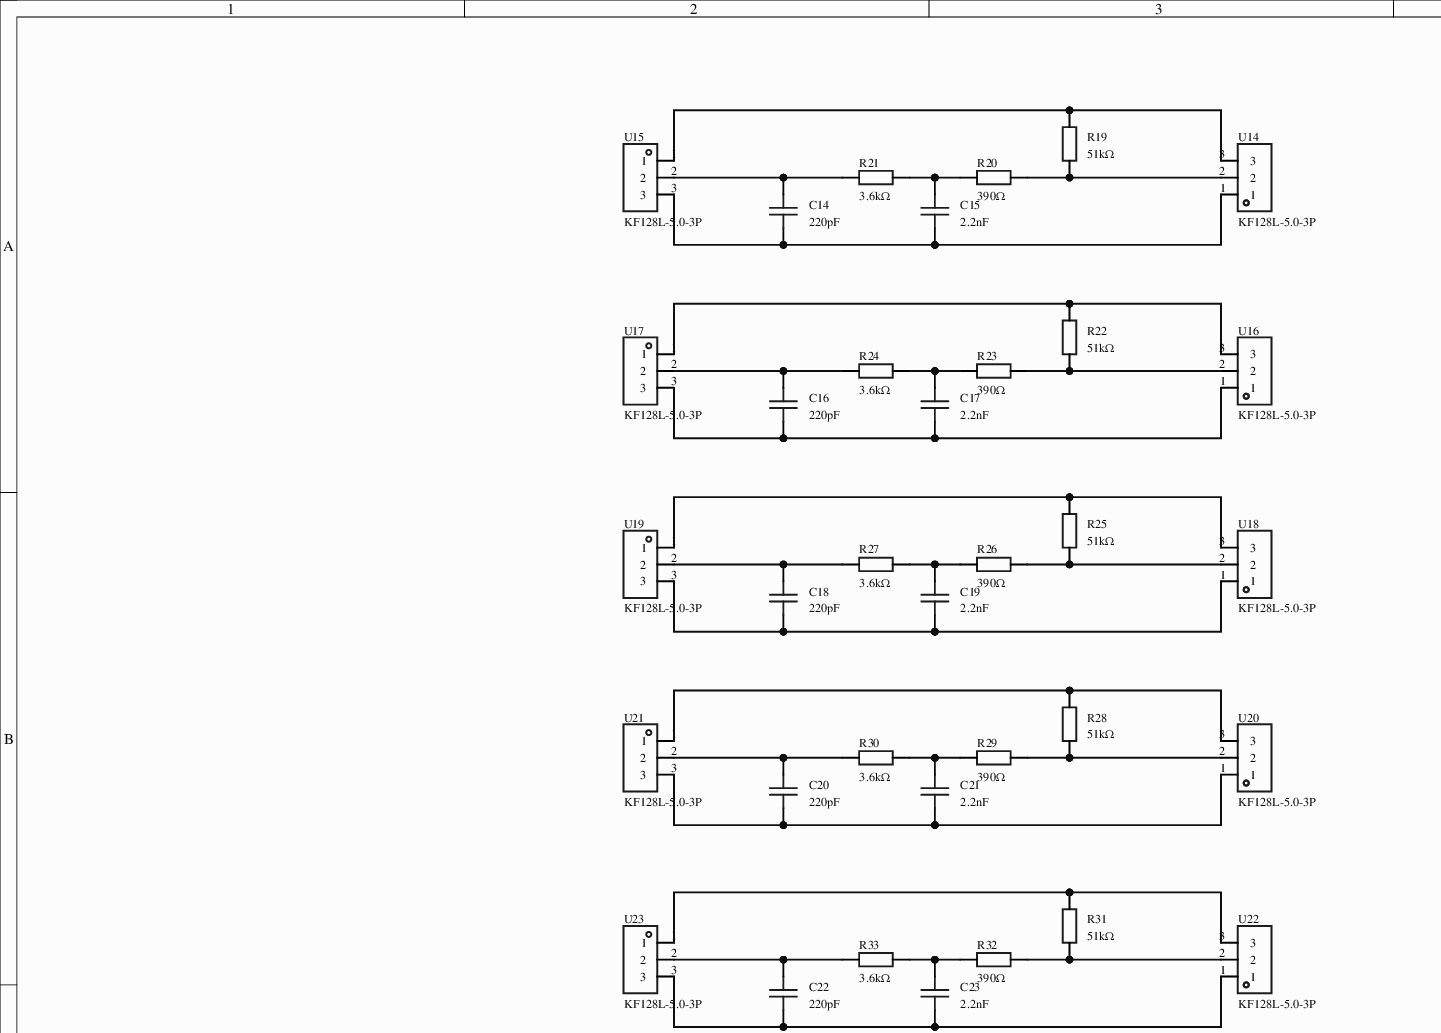
[diagram p0: MISC52118-3.schdoc, top left]
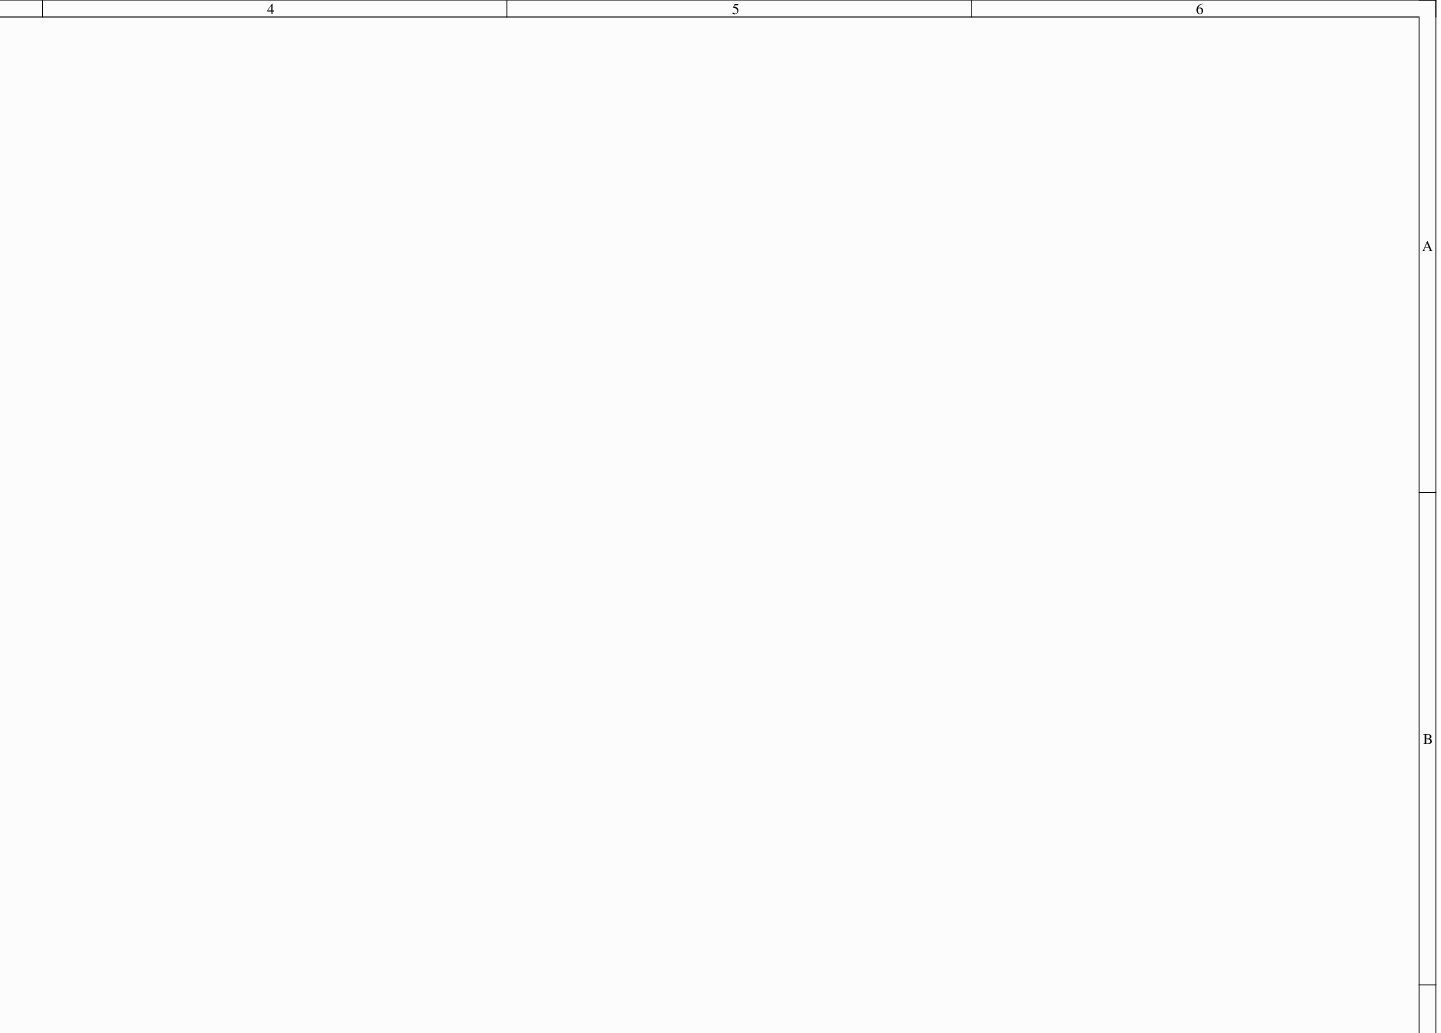
[diagram p1: MISC52118-3.schdoc, top right]
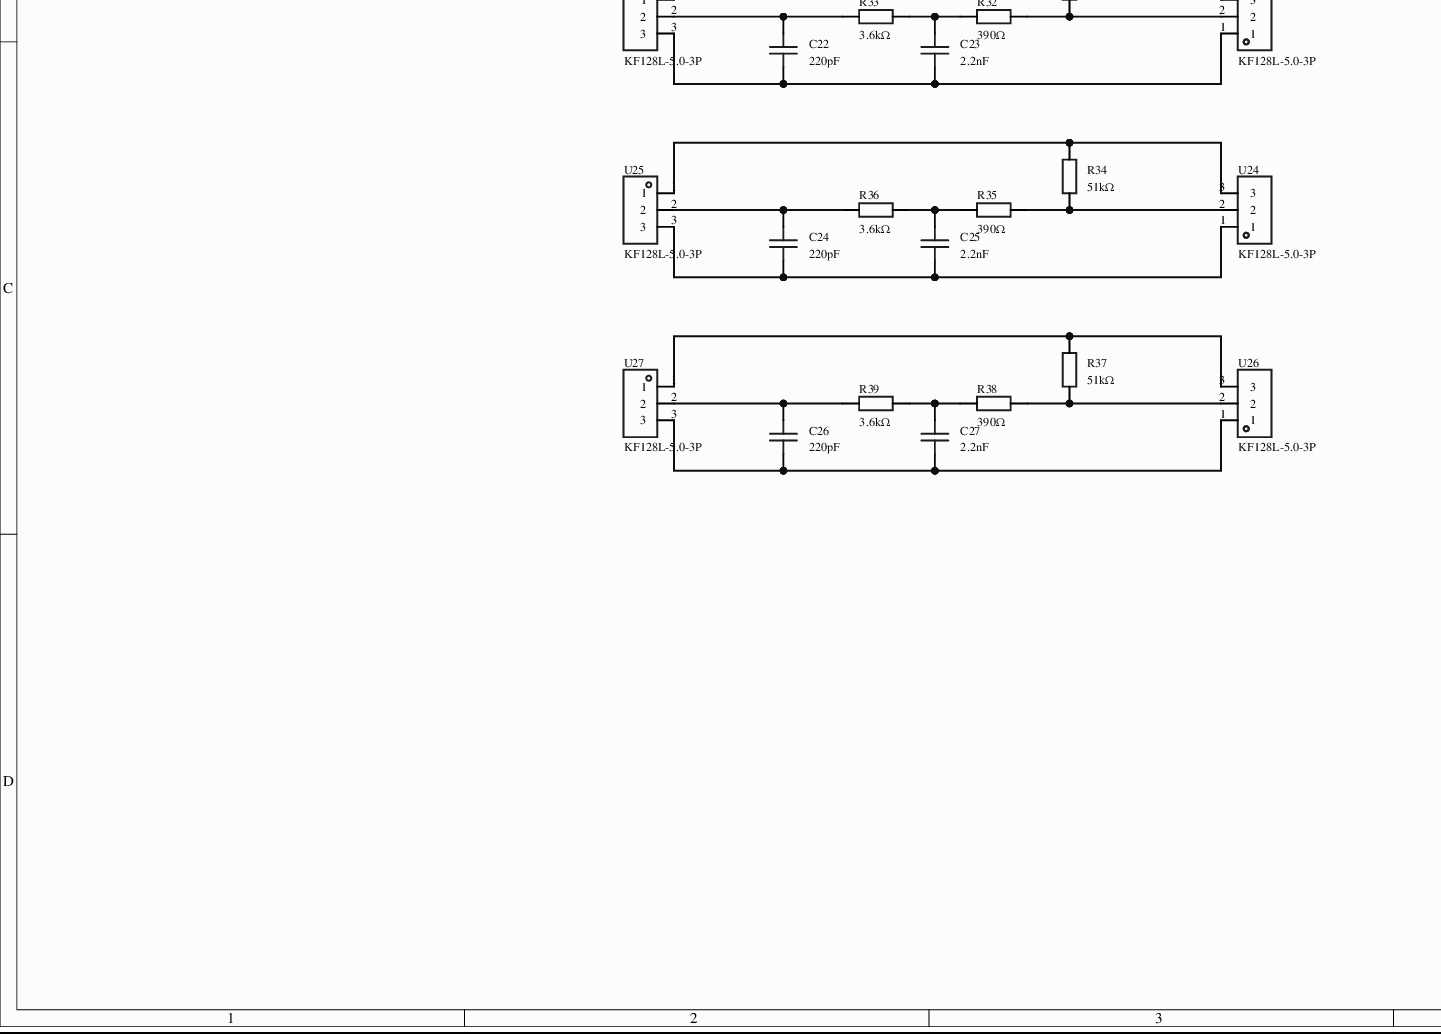
[diagram p2: MISC52118-3.schdoc, bottom left]
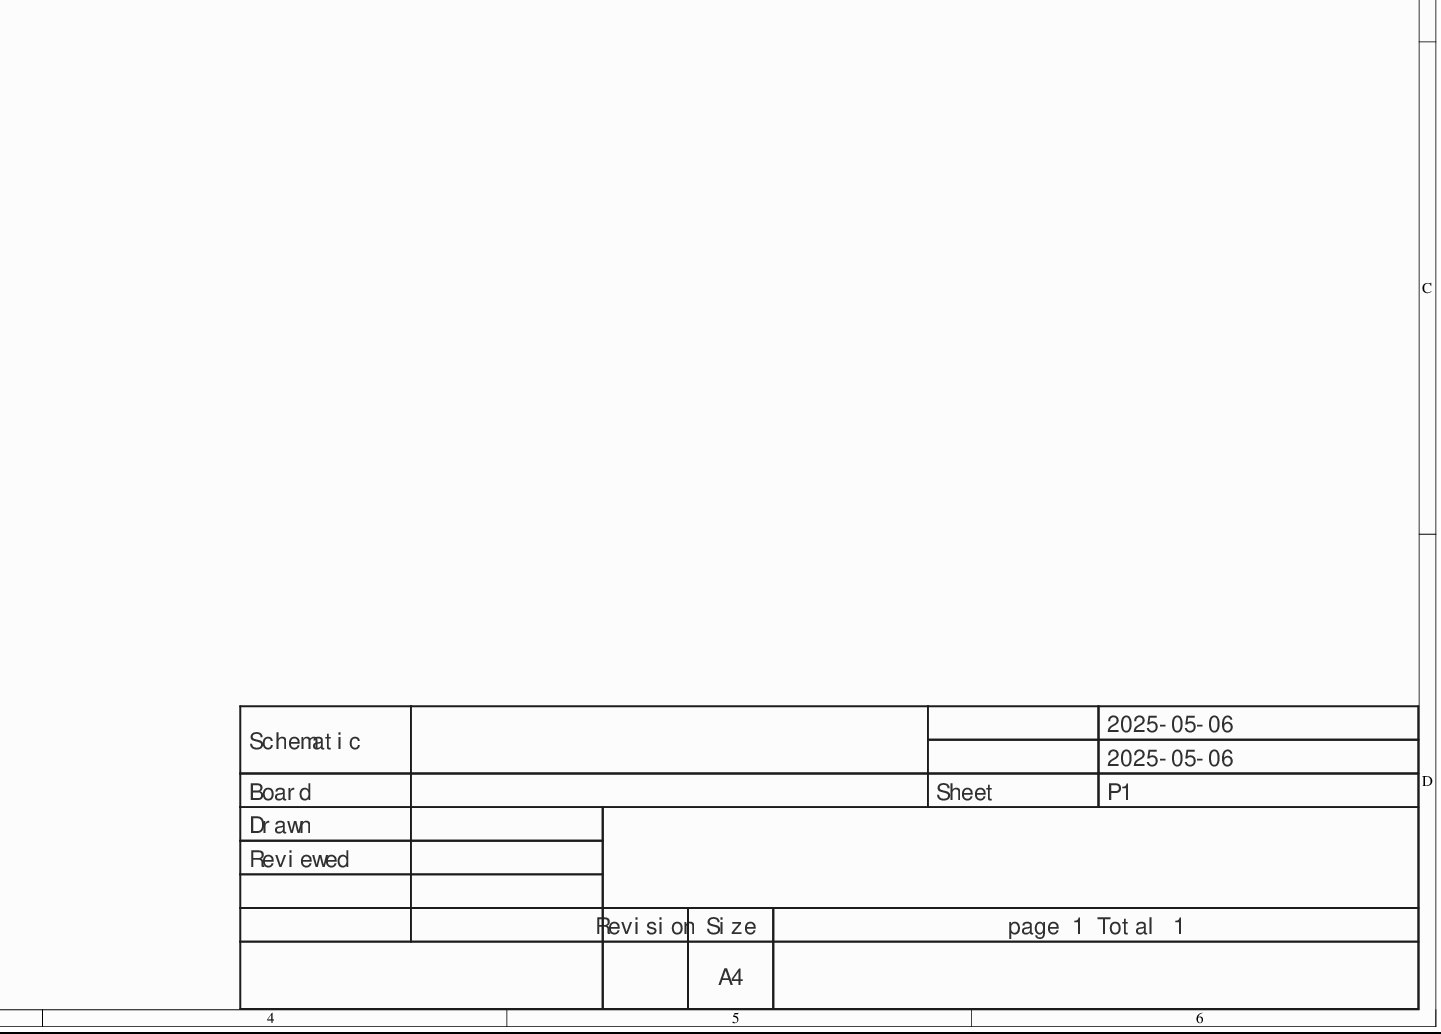
[diagram p3: MISC52118-3.schdoc, bottom right]
# Altium project MISC52118-2.PrjPcb
1 sheet, 49 parts. Net scope: global (net labels, ports and power ports of the same name join across sheets).
Board file: MISC52118.pcbdoc

## Sheet MISC52118-3.schdoc
size 420 x 297 mm; Version: V1.0; @Project Name: MISC52118; @Page Count: 1; @Update Date: 2025-05-06; @Create Date: 2025-05-06; @Schematic Name: MISC52118; @Page No: 1; @Create Time: 15:06:36; @Update Time: 15:06:39; @Board Name: MISC52118

### Parts
C14  220pF  [CAP-TH_L7.2-W4.5-P5.00-D0.5]
C15  2.2nF  [CAP-TH_L8.0-W5.0-P7.50-D1.0]
C16  220pF  [CAP-TH_L7.2-W4.5-P5.00-D0.5]
C17  2.2nF  [CAP-TH_L8.0-W5.0-P7.50-D1.0]
C18  220pF  [CAP-TH_L7.2-W4.5-P5.00-D0.5]
C19  2.2nF  [CAP-TH_L8.0-W5.0-P7.50-D1.0]
C20  220pF  [CAP-TH_L7.2-W4.5-P5.00-D0.5]
C21  2.2nF  [CAP-TH_L8.0-W5.0-P7.50-D1.0]
C22  220pF  [CAP-TH_L7.2-W4.5-P5.00-D0.5]
C23  2.2nF  [CAP-TH_L8.0-W5.0-P7.50-D1.0]
C24  220pF  [CAP-TH_L7.2-W4.5-P5.00-D0.5]
C25  2.2nF  [CAP-TH_L8.0-W5.0-P7.50-D1.0]
C26  220pF  [CAP-TH_L7.2-W4.5-P5.00-D0.5]
C27  2.2nF  [CAP-TH_L8.0-W5.0-P7.50-D1.0]
R19  51kΩ  [Res_1/4W]
R20  390Ω  [Res_1/4W]
R21  3.6kΩ  [Res_1/4W]
R22  51kΩ  [Res_1/4W]
R23  390Ω  [Res_1/4W]
R24  3.6kΩ  [Res_1/4W]
R25  51kΩ  [Res_1/4W]
R26  390Ω  [Res_1/4W]
R27  3.6kΩ  [Res_1/4W]
R28  51kΩ  [Res_1/4W]
R29  390Ω  [Res_1/4W]
R30  3.6kΩ  [Res_1/4W]
R31  51kΩ  [Res_1/4W]
R32  390Ω  [Res_1/4W]
R33  3.6kΩ  [Res_1/4W]
R34  51kΩ  [Res_1/4W]
R35  390Ω  [Res_1/4W]
R36  3.6kΩ  [Res_1/4W]
R37  51kΩ  [Res_1/4W]
R38  390Ω  [Res_1/4W]
R39  3.6kΩ  [Res_1/4W]
U14  KF128L-5.0-3P  [CONN-TH_3P-P5.00_KF128L-5.0-3P]
U15  KF128L-5.0-3P  [CONN-TH_3P-P5.00_KF128L-5.0-3P]
U16  KF128L-5.0-3P  [CONN-TH_3P-P5.00_KF128L-5.0-3P]
U17  KF128L-5.0-3P  [CONN-TH_3P-P5.00_KF128L-5.0-3P]
U18  KF128L-5.0-3P  [CONN-TH_3P-P5.00_KF128L-5.0-3P]
U19  KF128L-5.0-3P  [CONN-TH_3P-P5.00_KF128L-5.0-3P]
U20  KF128L-5.0-3P  [CONN-TH_3P-P5.00_KF128L-5.0-3P]
U21  KF128L-5.0-3P  [CONN-TH_3P-P5.00_KF128L-5.0-3P]
U22  KF128L-5.0-3P  [CONN-TH_3P-P5.00_KF128L-5.0-3P]
U23  KF128L-5.0-3P  [CONN-TH_3P-P5.00_KF128L-5.0-3P]
U24  KF128L-5.0-3P  [CONN-TH_3P-P5.00_KF128L-5.0-3P]
U25  KF128L-5.0-3P  [CONN-TH_3P-P5.00_KF128L-5.0-3P]
U26  KF128L-5.0-3P  [CONN-TH_3P-P5.00_KF128L-5.0-3P]
U27  KF128L-5.0-3P  [CONN-TH_3P-P5.00_KF128L-5.0-3P]

### Nets
NetC14_1: C14.1 C15.1 U14.1 U15.3
NetC14_2: C14.2 R21.2 U15.2
NetC15_2: C15.2 R20.2 R21.1
NetC16_1: C16.1 C17.1 U16.1 U17.3
NetC16_2: C16.2 R24.2 U17.2
NetC17_2: C17.2 R23.2 R24.1
NetC18_1: C18.1 C19.1 U18.1 U19.3
NetC18_2: C18.2 R27.2 U19.2
NetC19_2: C19.2 R26.2 R27.1
NetC20_1: C20.1 C21.1 U20.1 U21.3
NetC20_2: C20.2 R30.2 U21.2
NetC21_2: C21.2 R29.2 R30.1
NetC22_1: C22.1 C23.1 U22.1 U23.3
NetC22_2: C22.2 R33.2 U23.2
NetC23_2: C23.2 R32.2 R33.1
NetC24_1: C24.1 C25.1 U24.1 U25.3
NetC24_2: C24.2 R36.2 U25.2
NetC25_2: C25.2 R35.2 R36.1
NetC26_1: C26.1 C27.1 U26.1 U27.3
NetC26_2: C26.2 R39.2 U27.2
NetC27_2: C27.2 R38.2 R39.1
NetR19_1: R19.1 R20.1 U14.2
NetR19_2: R19.2 U14.3 U15.1
NetR22_1: R22.1 R23.1 U16.2
NetR22_2: R22.2 U16.3 U17.1
NetR25_1: R25.1 R26.1 U18.2
NetR25_2: R25.2 U18.3 U19.1
NetR28_1: R28.1 R29.1 U20.2
NetR28_2: R28.2 U20.3 U21.1
NetR31_1: R31.1 R32.1 U22.2
NetR31_2: R31.2 U22.3 U23.1
NetR34_1: R34.1 R35.1 U24.2
NetR34_2: R34.2 U24.3 U25.1
NetR37_1: R37.1 R38.1 U26.2
NetR37_2: R37.2 U26.3 U27.1

### Notes on the sheet
- 2025-05-06
- Schematic
- Board
- Sheet
- P1
- Drawn
- Reviewed
- Revision
- Size
- A4
- page 1 Total 1

### Library data of the parts
C14 C16 C18 C20 C22 C24 C26 = KP1830122633: Capacitance:220pF;Tolerance:±2.5%;Rated voltage:630V; 250V;Operating temperature:-55℃~+100℃;; Manufacturer: VISHAY(威世); AddInBom: yes; ModelId: 5b8f94d09378482e8a7d7c1f412bd9bb; ModelTransform: 283.464,177.165,0,0,0,0,0,0,-196.85; Tolerance: ±2.5%; Symbol: KP1830122633; Device: KP1830122633; LCSC Part Name: 220pF ±2.5% 630V 250V; SupplierPart: C3794724; ManufacturerPart: KP1830122633; Supplier Footprint: 插件,P=5mm; JLCPCB Part Class: Extended library; Datasheet: https://example.com/upload/public/pdf/source/20231212/3165E97C240197E63CE9BCA704937F9C.pdf; Supplier: LCSC; ConvertToPcb: yes; FootprintName: CAP-TH_L7.2-W4.5-P5.00-D0.5; ModelName: CAP-TH_L7.2-W4.5-P5.00-D0.5; Value: 220pF; Voltage Rated: 630V; 250V; Operating Temperature: -55℃~+100℃
C15 C17 C19 C21 C23 C25 C27 = DE2E3KY222MA3BU02F: Capacitance:2.2nF;Tolerance:±20%;Voltage(AC):300V;Class:X1,Y2;; Manufacturer: muRata(村田); AddInBom: yes; ModelId: 891483702e3d4cd188688a4834031f3d; ModelName: CAP-TH_L8.0-W5.0-H11.0-P7.0; ModelTransform: 314.96,196.85,0,0,0,0,0,0,-137.795; Tolerance: ±20%; Voltage(AC): 300V; Subclass: X1,Y2; Symbol: DE2E3KY222MA3BU02F; Device: DE2E3KY222MA3BU02F; LCSC Part Name: 等级:X1,Y2 2.2nF ±20% 300V; SupplierPart: C237450; ManufacturerPart: DE2E3KY222MA3BU02F; Supplier Footprint: 插件,P=7.5mm; JLCPCB Part Class: Extended library; Datasheet: https://example.com/upload/public/pdf/source/20191022/C440140_7AB5F4B3B56EC7AEB2A782F4DBA79A52.pdf; Supplier: LCSC; ConvertToPcb: yes; FootprintName: CAP-TH_L8.0-W5.0-P7.50-D1.0; Value: 2.2nF; Operating Temperature: -40℃~+125℃
R19-R39 = Res_AXIAL-1/4W: AddInBom: yes; SymbolName: Resistor; ModelId: 463263665006444ab7a47bd11b0cf956; ModelName: RES-TH_BD2.4-L6.3-P10.30-D0.6; ModelTransform: 427.165,94.32816,0,0,0,0,0,0,-196.85; Device: Res_AXIAL-1/4W; Supplier Footprint: 轴向引线; ConvertToPcb: yes; FootprintName: Res_1/4W
  R19 R22 R25 R28 R31 R34 R37: Value: 51kΩ
  R20 R23 R26 R29 R32 R35 R38: Value: 390Ω
  R21 R24 R27 R30 R33 R36 R39: Value: 3.6kΩ
U14-U27 = KF128L-5.0-3P: Stackable copper RoHS; Manufacturer: KEFA(科发); AddInBom: yes; ModelId: cc3e985db2e2444581f9de0f33be2442; ModelTransform: 602.361,393.7,0,0,0,0,5.906,-3.937,-169.291; Symbol: KF128L-5.0-3P; Device: KF128L-5.0-3P; LCSC Part Name: 间距P=5.0mm 3Pin位 直插 直针 可拼接 铜 环保; SupplierPart: C474939; ManufacturerPart: KF128L-5.0-3P; Supplier Footprint: P=5mm; JLCPCB Part Class: Extended library; Datasheet: https://example.com/upload/public/pdf/source/20230317/752C0AC053DC32F5BE41F95D5E9BCBBC.pdf; Supplier: LCSC; ConvertToPcb: yes; FootprintName: CONN-TH_3P-P5.00_KF128L-5.0-3P; ModelName: CONN-TH_3P-P5.00_KF128L-5.0-3P